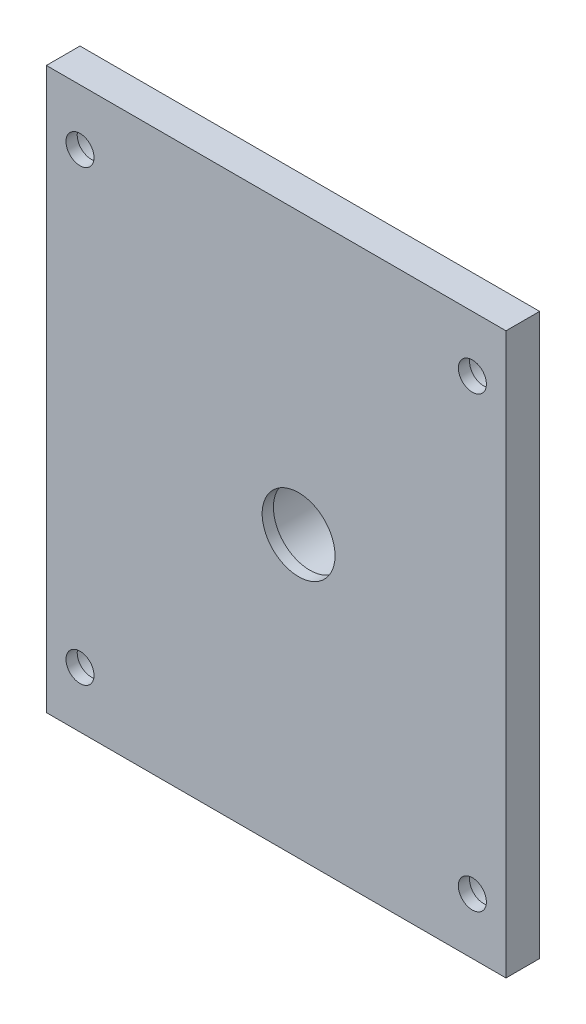
SolidWorks part; units mm, degrees
ref_plane "前视基准面" through (0, 0, 0) normal (0, 0, 1) x (1, 0, 0)
ref_plane "上视基准面" through (0, 0, 0) normal (0, 1, 0) x (1, 0, 0)
ref_plane "右视基准面" through (0, 0, 0) normal (1, 0, 0) x (0, 0, -1)
other "Configuration Table"
sketch "草图1" plane through (0, 0, 0) normal (0, 0, 1) x (1, 0, 0)
  line L0 (-64.3373, 0) -> (70.6024, 0) construction
  line L1 (0, 86.3855) -> (0, -84.4578) construction
  line L2 (-41, 63.7349) -> (-41, -72.4096) construction
  line L3 (-79.0361, 50) -> (91.3253, 50) construction
  line L4 (41, 50) -> (-41, 50)
  line L5 (-41, 50) -> (-41, -50)
  line L6 (41, 50) -> (41, -50)
  line L7 (41, -50) -> (-41, -50)
  point P14 (0, 50)
  point P15 (-41, 0)
  dimension "D1" = 50
  dimension "D2" = 41
extrude "凸台-拉伸1" add sketch "草图1" along normal blind 6
sketch "草图3" plane through (0, 0, 6) normal (0, 0, 1) x (1, 0, 0)
  line L0 (-60.9017, 0) -> (63.8991, 0) construction
  line L1 (4, 54.1575) -> (4, -54.1575) construction
  line L2 (-41, 50) -> (-41, -50) construction
  circle A0 centre (4, 0) radius 12
  dimension "D2" = 24
  dimension "D1" = 45
extrude "凸台-拉伸3" add sketch "草图3" against normal blind 14
sketch "草图5" plane through (0, 0, 6) normal (0, 0, 1) x (1, 0, 0)
  line L0 (-62.4004, 0) -> (79.2948, 0) construction
  line L1 (4, 54.43) -> (4, -54.43) construction
  line L2 (-41, 50) -> (-41, -50) construction
  circle A0 centre (4, 0) radius 6.5
  dimension "D2" = 13
  dimension "D1" = 45
sketch "草图7" plane through (0, 0, 0) normal (0, 0, -1) x (-1, 0, 0)
  line L0 (-73.0275, 0) -> (67.8502, 0) construction
  line L1 (0, 63.9015) -> (0, -60.3458) construction
  line L2 (-35, 59.342) -> (-35, 28.5651) construction
  line L3 (-41, -50) -> (-41, 50) construction
  line L4 (-44.8045, 40) -> (-3.7687, 40) construction
  line L5 (-41, 50) -> (41, 50) construction
  circle A0 centre (-35, 40) radius 4
  circle A1 centre (-35, -40) radius 4
  circle A2 centre (35, -40) radius 4
  circle A3 centre (35, 40) radius 4
  dimension "D3" = 8
  dimension "D1" = 6
  dimension "D2" = 10
extrude "切除-拉伸4" cut sketch "草图7" against normal blind 4
extrude "切除-拉伸8" cut sketch "草图5" against normal blind 2
sketch "草图11" plane through (0, 0, -8) normal (0, 0, -1) x (-1, 0, 0)
  circle A0 centre (-4, 0) radius 7.5
extrude "切除-拉伸9" cut sketch "草图11" against normal blind 12
sketch "草图12" plane through (0, 0, 0) normal (0, 0, -1) x (-1, 0, 0)
  line L0 (0, 52.1693) -> (0, -54.9316) construction
  line L1 (-60.8963, 0) -> (65.3011, 0) construction
  circle A0 centre (-35, -40) radius 2.5
  circle A1 centre (-35, 40) radius 2.5
  circle A2 centre (35, -40) radius 2.5
  circle A3 centre (35, 40) radius 2.5
extrude "切除-拉伸10" cut sketch "草图12" against normal blind 6
